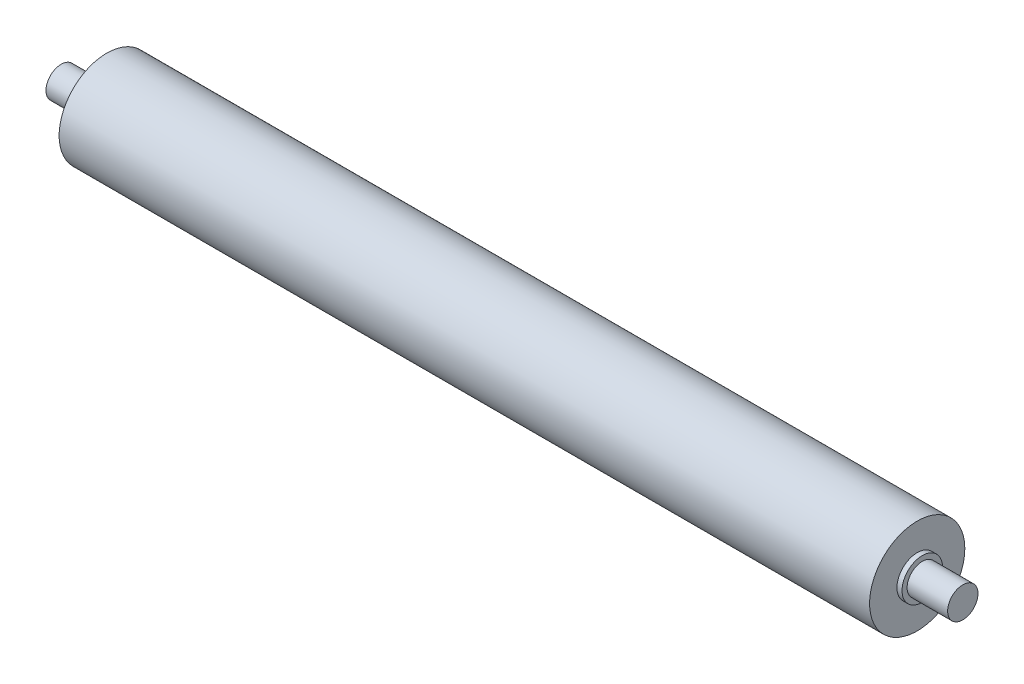
SolidWorks part; units mm, degrees
material "Q235"
ref_plane "Front" through (0, 0, 0) normal (0, 0, 1) x (1, 0, 0)
ref_plane "Top" through (0, 0, 0) normal (0, 1, 0) x (1, 0, 0)
ref_plane "Right" through (0, 0, 0) normal (1, 0, 0) x (0, 0, -1)
sketch "Sketch1" plane through (0, 0, 0) normal (0, 0, 1) x (1, 0, 0)
  line L0 (0, 0) -> (0, 7.5)
  line L1 (0, 7.5) -> (20, 7.5)
  line L2 (20, 7.5) -> (20, 10)
  line L3 (20, 10) -> (22.5, 10)
  line L4 (22.5, 10) -> (22.5, 23.5)
  line L5 (22.5, 23.5) -> (422.5, 23.5)
  line L6 (222.5, 23.5) -> (222.5, 0) construction
  line L7 (445, 0) -> (0, 0)
  line L8 (422.5, 10) -> (422.5, 23.5)
  line L9 (425, 10) -> (422.5, 10)
  line L10 (425, 7.5) -> (425, 10)
  line L11 (445, 7.5) -> (425, 7.5)
  line L12 (445, 0) -> (445, 7.5)
  line L13 (0, 0) -> (-5.488, 0) construction
  dimension "D1" = 47
  dimension "D2" = 15
  dimension "D3" = 20
  dimension "D4" = 400
  dimension "D5" = 2.5
  dimension "D6" = 20
revolve "Revolve1" add sketch "Sketch1" angle 360 about L13
